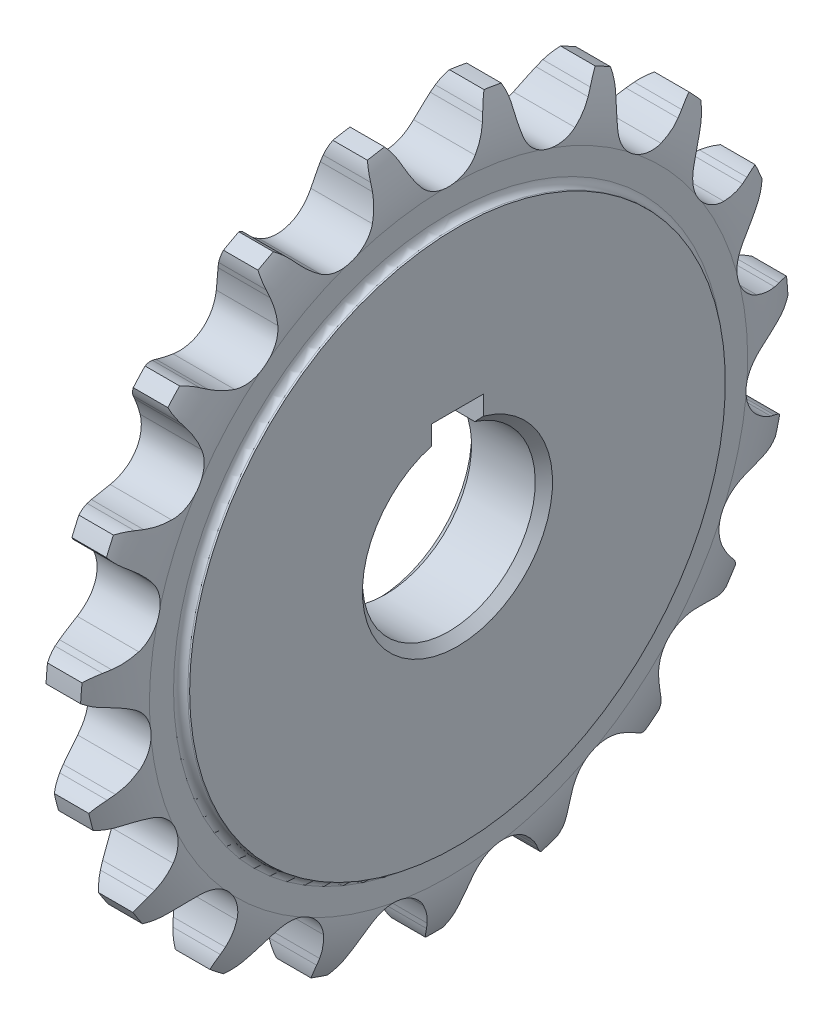
SolidWorks part; units mm, degrees
ref_plane "前视基准面" through (0, 0, 0) normal (0, 0, 1) x (1, 0, 0)
ref_plane "上视基准面" through (0, 0, 0) normal (0, 1, 0) x (1, 0, 0)
ref_plane "右视基准面" through (0, 0, 0) normal (1, 0, 0) x (0, 0, -1)
sketch "草图1" plane through (0, 0, 0) normal (0, 0, 1) x (1, 0, 0)
  line L0 (-6.35, 0) -> (6.35, 0) construction
  line L1 (-4.6852, 10) -> (-4.6852, 31)
  line L2 (-4.6852, 31) -> (-4.4782, 31)
  line L3 (-3.6502, 31.8279) -> (-3.6502, 34.6196)
  line L4 (-1.9992, 41) -> (1.9992, 41)
  line L5 (3.6502, 34.6196) -> (3.6502, 31.8279)
  line L6 (4.4782, 31) -> (4.6852, 31)
  line L7 (4.6852, 31) -> (4.6852, 10)
  line L8 (4.6852, 10) -> (-4.6852, 10)
  line L9 (0, 0) -> (0, 41) construction
  line L10 (-3.0556, 38.5796) -> (3.0556, 38.5796) construction
  line L11 (-3.0556, -38.5796) -> (3.0556, -38.5796) construction
  line L12 (6.35, 0) -> (25.35, 0) construction
  line L13 (-3.6502, 34.6196) -> (3.7984, 34.6196) construction
  line L14 (-3.6502, -34.6196) -> (3.7984, -34.6196) construction
  line L15 (25.35, 0) -> (33.27, 0) construction
  line L16 (33.27, 0) -> (45.34, 0) construction
  line L17 (45.34, 0) -> (53.19, 0) construction
  line L18 (53.19, 0) -> (67.57, 0) construction
  arc A0 (-1.9992, 41) -> (-3.6502, 34.6196) centre (9.0492, 34.7373) ccw
  arc A1 (1.9992, 41) -> (3.6502, 34.6196) centre (-9.0492, 34.7373) cw
  arc A2 (3.6502, 31.8279) -> (4.4782, 31) centre (4.4782, 31.8279) ccw
  arc A3 (-4.4782, 31) -> (-3.6502, 31.8279) centre (-4.4782, 31.8279) ccw
  point P30 (3.6502, 31)
  point P33 (-3.6502, 31)
  dimension "D1" = 3.6196
  dimension "rx" = 12.7
  dimension "D3" = 0.8279
  dimension "d" = 77.1593
  dimension "p" = 12.7
  dimension "z" = 19
  dimension "da" = 82
  dimension "df" = 69.2393
  dimension "dr" = 7.92
  dimension "dk" = 20
  dimension "dg" = 62
  dimension "h" = 12.07
  dimension "bf1" = 7.3005
  dimension "b1" = 7.85
  dimension "ba" = 1.651
  dimension "D2" = 1.0349
  dimension "pt" = 14.38
revolve "旋转1" add sketch "草图1" angle 360 about L0
sketch "草图2" plane through (0, 0, 0) normal (1, 0, 0) x (0, 0, -1)
  line L0 (0, 0) -> (0, 41) construction
  line L1 (0, 0) -> (-6.7484, 40.4408) construction
  line L2 (0, 0) -> (-13.3127, 38.7785) construction
  line L3 (3.1687, 36.0899) -> (3.1879, 36.0748) construction
  line L4 (4.5522, 38.4265) -> (-4.9821, 42.4942) construction
  line L5 (0, 0) -> (6.7484, 40.4408) construction
  line L6 (4.5522, 38.4265) -> (4.8587, 39.1448)
  line L7 (-4.5522, 38.4265) -> (-4.8587, 39.1448)
  circle A0 centre (0, 0) radius 41 construction
  arc A1 (3.1687, 36.0899) -> (-3.1687, 36.0899) centre (0, 38.5796) cw
  arc A2 (3.1687, 36.0899) -> (4.5522, 38.4265) centre (-4.9821, 42.4942) ccw
  arc A3 (5.7509, 40.5947) -> (4.8587, 39.1448) centre (10.1556, 36.885) ccw
  arc A4 (-3.1687, 36.0899) -> (-4.5522, 38.4265) centre (4.9821, 42.4942) cw
  arc A5 (-5.7509, 40.5947) -> (-4.8587, 39.1448) centre (-10.1556, 36.885) cw
  arc A7 (5.7509, 40.5947) -> (-5.7509, 40.5947) centre (0, 0) ccw
  dimension "r1" = 4.0298
  dimension "r3" = 5.7588
  dimension "D1" = 18.947
  dimension "D2" = 9.474
  dimension "α/2" = 51.842
  dimension "M" = 4.9821
  dimension "T" = 3.9146
  dimension "β" = 15.053
  dimension "γ/2" = 13.632
  dimension "bc" = 0.781
extrude "切除-拉伸1" cut sketch "草图2" against normal mid plane 9.3703
pattern_circular "阵列(圆周)1" count 19 over 360 about axis through (0, 0, 0) along (1, 0, 0) of "切除-拉伸1"
sketch "草图3" plane through (0, 0, 0) normal (0, 0, 1) x (1, 0, 0)
  line L0 (4.6852, 10) -> (10.3148, 10)
  line L3 (10.3148, 10) -> (10.3148, 18.9049)
  line L4 (10.3148, 18.9049) -> (4.6852, 18.9049)
  line L5 (4.6852, 18.9049) -> (4.6852, 10)
  line L6 (0, 0) -> (4.8, 0) construction
  line L8 (-4.6852, 31) -> (-4.6852, -31) construction
  dimension "h" = 8.9049
  dimension "K" = 4.8
  dimension "L" = 15
revolve "旋转2" [suppressed] add sketch "草图3" angle 360 about L6
sketch "草图4" plane through (-4.6852, 0, 0) normal (-1, 0, 0) x (0, 0, 1)
  line L1 (-3, 9.5394) -> (3, 9.5394)
  line L2 (-3, 9.5394) -> (-3, 12.8)
  line L3 (-3, 12.8) -> (3, 12.8)
  line L4 (3, 9.5394) -> (3, 12.8)
  circle A0 centre (0, 0) radius 10 construction
  point P6 (0.2, 12.8)
  dimension "D1" = 12.8
  dimension "键槽宽度" = 6
  dimension "t1" = 2.8
extrude "切除-拉伸2" cut sketch "草图4" against normal through all
chamfer "倒角1" distance 1 angle 45 1 edges at (-4.6852, -10, 0)
chamfer "倒角2" distance 1 angle 45 1 edges at (4.6852, -10, 0)
chamfer "倒角3" [suppressed] distance 1 angle 45
